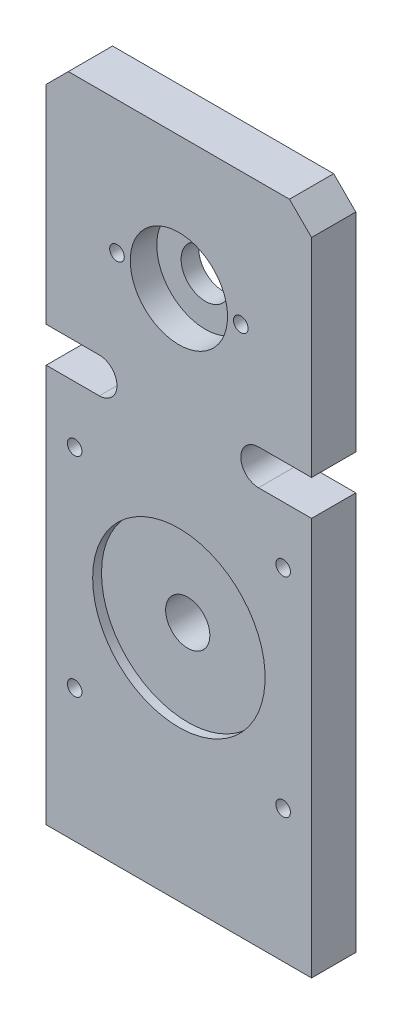
from build123d import *

# Parameters (mm, degrees)
SKETCH1_W             = 60
SKETCH1_H             = 150
BOSS_EXTRUDE1_DEPTH   = 10
CHAMFER1_SIZE         = 5
CUT_EXTRUDE5_START    = -10
SKETCH5_R             = 19.5
CUT_EXTRUDE5_DEPTH    = 2
SKETCH6_R             = 5
CUT_EXTRUDE6_DEPTH    = 82.172655494
M4_TAPPED_HOLE1_D     = 3.3
SKETCH9_R             = 11
CUT_EXTRUDE7_DEPTH    = 6
SKETCH10_R            = 5.5
CUT_EXTRUDE8_DEPTH    = 82
CUT_EXTRUDE9_DEPTH    = 82.39410298
M4_TAPPED_HOLE2_D     = 3.3
M4_TAPPED_HOLE3_D     = 3.3
M4_TAPPED_HOLE3_DEPTH = 11.5
M4_TAPPED_HOLE3_TIP   = 0.991420021


with BuildPart() as part:
    # Sketch1 → Boss-Extrude1 (new body)
    with BuildSketch(Plane.XY):
        Rectangle(SKETCH1_W, SKETCH1_H)
    extrude(amount=BOSS_EXTRUDE1_DEPTH)

    # Chamfer1
    chamfer1_edges = [part.edges().sort_by_distance(p)[0] for p in [
        (-30, 75, 5),
        (30, 75, 5),
    ]]
    chamfer(chamfer1_edges, length=CHAMFER1_SIZE)

    # Sketch5 → Cut-Extrude5 (cut)
    with BuildSketch(Plane(origin=(0, 0, 0), x_dir=(-1, 0, 0), z_dir=(0, 0, -1)).offset(CUT_EXTRUDE5_START)):
        with Locations((0, -21.425)):
            Circle(SKETCH5_R)
    extrude(amount=CUT_EXTRUDE5_DEPTH, mode=Mode.SUBTRACT)

    # Sketch6 → Cut-Extrude6 (cut, through all)
    with BuildSketch(Plane.XY.offset(8)):
        with Locations((0, -21.425)):
            Circle(SKETCH6_R)
    extrude(amount=-CUT_EXTRUDE6_DEPTH, mode=Mode.SUBTRACT)

    # M4 Tapped Hole1 (through all)
    with Locations(Plane.XY.offset(10)):
        with Locations((-23.57, 2.145), (-23.57, -44.995), (23.57, 2.145), (23.57, -44.995)):
            Hole(M4_TAPPED_HOLE1_D / 2)

    # Sketch9 → Cut-Extrude7 (cut)
    with BuildSketch(Plane.XY.offset(10)):
        with Locations((0, 45)):
            Circle(SKETCH9_R)
    extrude(amount=-CUT_EXTRUDE7_DEPTH, mode=Mode.SUBTRACT)

    # Sketch10 → Cut-Extrude8 (cut, through all)
    with BuildSketch(Plane.XY.offset(4)):
        with Locations((0, 45)):
            Circle(SKETCH10_R)
    extrude(amount=-CUT_EXTRUDE8_DEPTH, mode=Mode.SUBTRACT)

    # Sketch11 → Cut-Extrude9 (cut, through all)
    with BuildSketch(Plane(origin=(0, 0, 0), x_dir=(-1, 0, 0), z_dir=(0, 0, -1))):
        with BuildLine():
            Line((18, 23), (40.992730917, 23))
            ThreePointArc((40.992730917, 23), (44.992730917, 19), (40.992730917, 15))
            Line((40.992730917, 15), (18, 15))
            ThreePointArc((18, 15), (14, 19), (18, 23))
        make_face()
    cut_extrude9 = extrude(amount=-CUT_EXTRUDE9_DEPTH, mode=Mode.SUBTRACT)

    # Mirror1: Cut-Extrude9 across plane
    add(cut_extrude9.mirror(Plane(origin=(0, 0, 0), x_dir=(0, 0, 1), z_dir=(1, 0, 0))), mode=Mode.SUBTRACT)

    # M4 Tapped Hole2 (through all)
    with Locations(Plane.XY.offset(10)):
        with Locations((-14, 45), (14, 45)):
            Hole(M4_TAPPED_HOLE2_D / 2)

    # M4 Tapped Hole3
    with Locations(Plane(origin=(0, -75, 0), x_dir=(-1, 0, 0), z_dir=(0, -1, 0))):
        with Locations((20, -5), (-20, -5)):
            Hole(M4_TAPPED_HOLE3_D / 2, depth=M4_TAPPED_HOLE3_DEPTH)
            with Locations((0, 0, -(M4_TAPPED_HOLE3_DEPTH + M4_TAPPED_HOLE3_TIP / 2))):  # 118° drill point
                Cone(0, M4_TAPPED_HOLE3_D / 2, M4_TAPPED_HOLE3_TIP, mode=Mode.SUBTRACT)


solid = part.part
